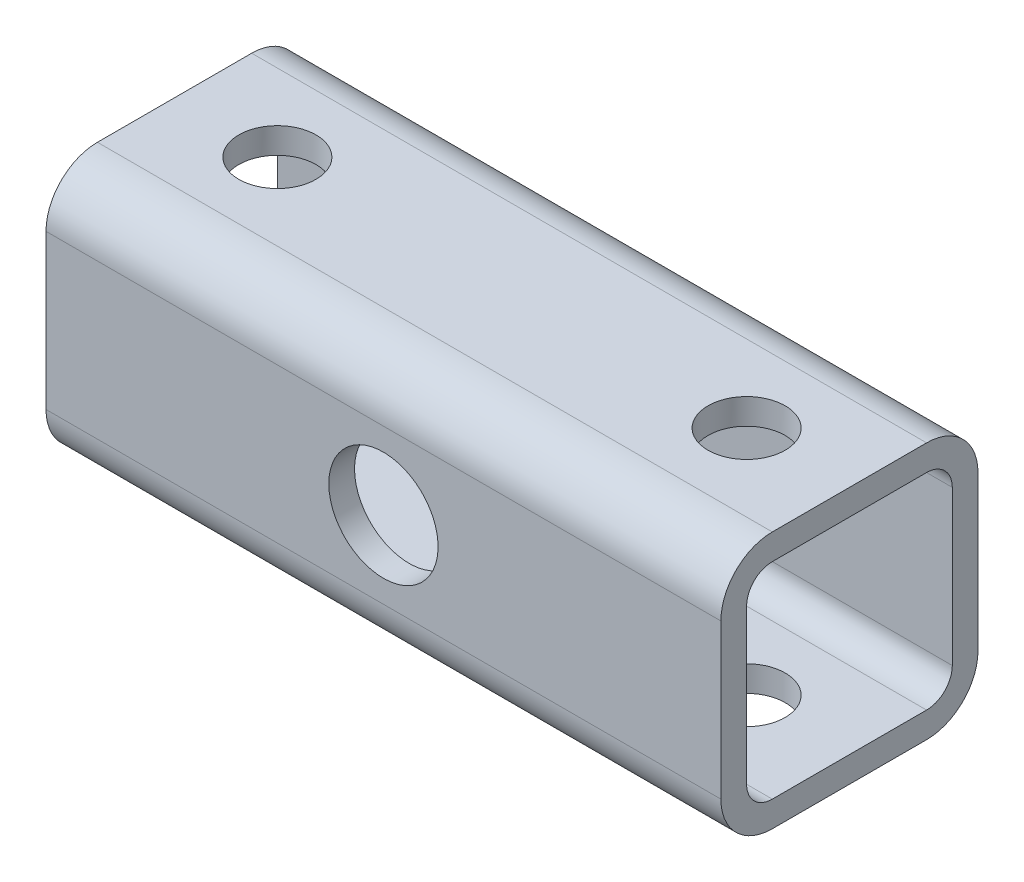
SolidWorks part; units mm, degrees
ref_plane "前视基准面" through (0, 0, 0) normal (0, 0, 1) x (1, 0, 0)
ref_plane "上视基准面" through (0, 0, 0) normal (0, 1, 0) x (1, 0, 0)
ref_plane "右视基准面" through (0, 0, 0) normal (1, 0, 0) x (0, 0, -1)
sketch "草图1" plane through (0, 0, 0) normal (0, 0, 1) x (1, 0, 0)
  line L0 (0, 0) -> (105, 0)
  dimension "D1" = 105
other "冷弯空心方管gb∕t6728-2002 40 X 40 X 4(1)"
ref_plane "基准面1" through (0, 0, 0) normal (1, 0, 0) x (0, 1, 0)
sketch "Sketch1" plane through (0, 0, 0) normal (1, 0, 0) x (0, 1, 0)
  line L0 (-12, -16) -> (12, -16)
  line L1 (-16, -12) -> (-16, 12)
  line L2 (12, 16) -> (-12, 16)
  line L3 (16, 12) -> (16, -12)
  line L4 (-12, -20) -> (12, -20)
  line L5 (-20, -12) -> (-20, 12)
  line L6 (12, 20) -> (-12, 20)
  line L7 (20, 12) -> (20, -12)
  arc A0 (20, 12) -> (12, 20) centre (12, 12) ccw
  arc A1 (12, -20) -> (20, -12) centre (12, -12) ccw
  arc A2 (-20, -12) -> (-12, -20) centre (-12, -12) ccw
  arc A3 (-12, 20) -> (-20, 12) centre (-12, 12) ccw
  arc A4 (-12, 16) -> (-16, 12) centre (-12, 12) ccw
  arc A5 (16, 12) -> (12, 16) centre (12, 12) ccw
  arc A6 (12, -16) -> (16, -12) centre (12, -12) ccw
  arc A7 (-16, -12) -> (-12, -16) centre (-12, -12) ccw
  point P0 (-20, 0)
  point P1 (20, 0)
  point P2 (0, 20)
  point P3 (0, -20)
  point P4 (0, 0)
  point P5 (-20, -20)
  point P6 (20, -20)
  point P7 (20, 20)
  point P8 (-20, 20)
  point P33 (0, 0)
  dimension "D1" = 8
  dimension "Thickness" = 4
  dimension "V_leg" = 40
hole_wizard "Ø12.0 (12) 直径孔1" positions "草图3" profile "草图4" hole size "Ø12.0" standard "GB"
sketch "草图3" plane through (0, 20, 0) normal (0, 1, 0) x (1, 0, 0)
  line L0 (0, 0) -> (105, 0) construction
  line L1 (105, 12) -> (105, -12) construction
  point P0 (16, 0)
  point P4 (89, 0)
  dimension "D1" = 16
  dimension "D2" = 16
sketch "草图4" plane through (16, 20, 0) normal (1, 0, 0) x (0, 0, 1)
  line L0 (0, 0) -> (0, 45)
  line L1 (0, 45) -> (6, 41.3948)
  line L2 (6, 41.3948) -> (6, 0)
  line L5 (6, 0) -> (0, 0)
  line L10 (0, 45) -> (-6, 41.3948) construction
  line L11 (0, -6.35) -> (0, 107.95) construction
  dimension "孔直径" = 12
  dimension "孔深度" = 45
  dimension "导头角度" = 118
sketch "草图5" plane through (0, 0, -20) normal (0, 0, -1) x (-1, 0, 0)
  line L0 (-105, -12) -> (-105, 12) construction
  circle A0 centre (-52.5, 0) radius 8.5
  dimension "D1" = 52.5
  dimension "D2" = 17
extrude "切除-拉伸1" cut sketch "草图5" against normal up to surface (40 mm away) up to face at (52.5, 0, 20)
